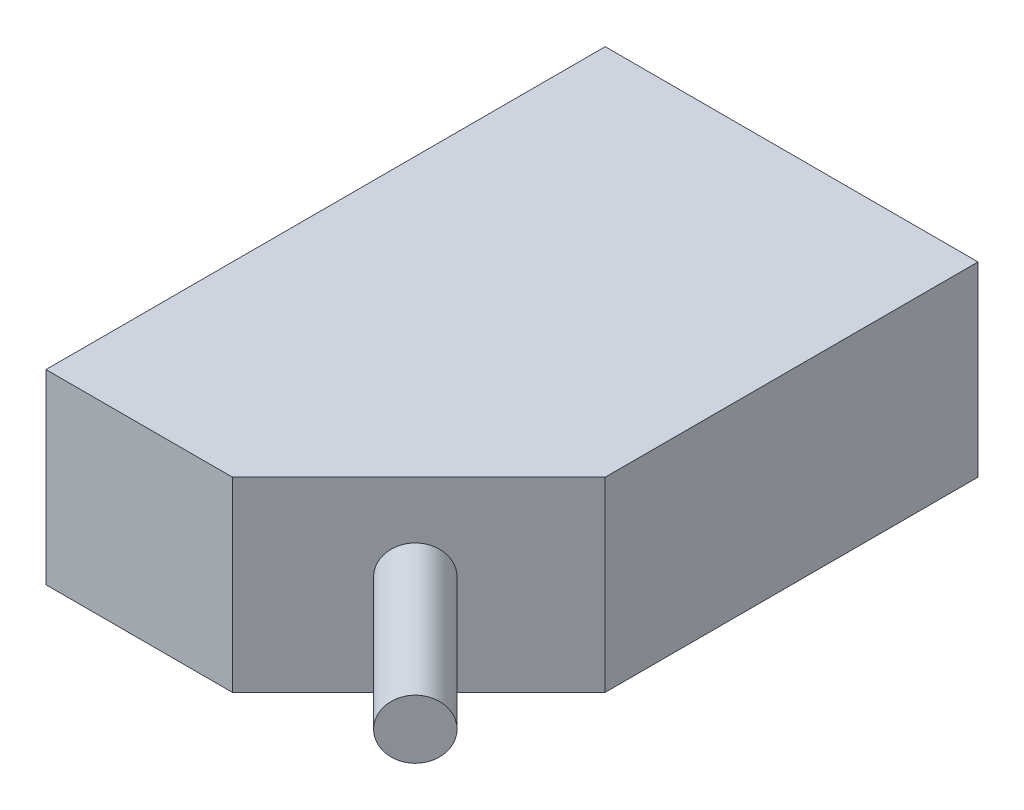
from build123d import *

# Parameters (mm, degrees)
SKETCH1_W           = 20
SKETCH1_H           = 30
BOSS_EXTRUDE1_DEPTH = 10
CHAMFER1_SIZE       = 10
SKETCH2_R           = 1.584264685
BOSS_EXTRUDE2_DEPTH = 10


with BuildPart() as part:
    # Sketch1 → Boss-Extrude1 (new body)
    with BuildSketch(Plane(origin=(0, 0, 0), x_dir=(1, 0, 0), z_dir=(0, 1, 0))):
        with Locations((10, -15)):
            Rectangle(SKETCH1_W, SKETCH1_H)
    extrude(amount=BOSS_EXTRUDE1_DEPTH)

    # Chamfer1
    chamfer1_edges = [part.edges().sort_by_distance(p)[0] for p in [
        (20, 5, 30),
    ]]
    chamfer(chamfer1_edges, length=CHAMFER1_SIZE)

    # Sketch2 → Boss-Extrude2 (add)
    with BuildSketch(Plane(origin=(20, 0, 20), x_dir=(0.7071067811865487, 0, -0.7071067811865465), z_dir=(0.7071067811865465, 0, 0.7071067811865487))):
        with Locations((-7.203605768, 5.360257058)):
            Circle(SKETCH2_R)
    extrude(amount=BOSS_EXTRUDE2_DEPTH)


solid = part.part
